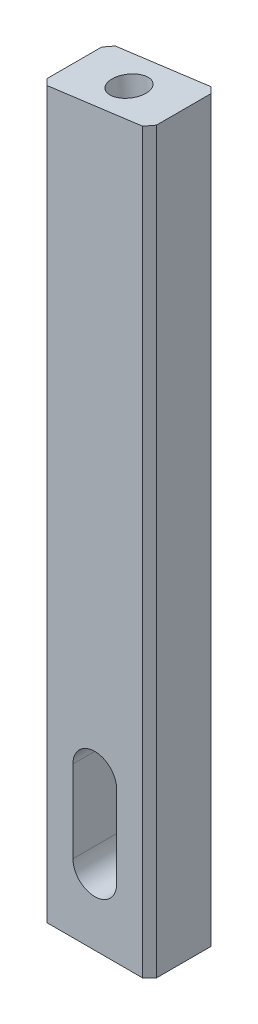
SolidWorks part; units mm, degrees
ref_plane "Front Plane" through (0, 0, 0) normal (0, 0, 1) x (1, 0, 0)
ref_plane "Top Plane" through (0, 0, 0) normal (0, 1, 0) x (1, 0, 0)
ref_plane "Right Plane" through (0, 0, 0) normal (1, 0, 0) x (0, 0, -1)
sketch "Sketch1" plane through (0, 0, 0) normal (0, 0, 1) x (1, 0, 0)
  line L1 (-4, 27) -> (4, 27)
  line L2 (-4, 27) -> (-4, -27)
  line L3 (-4, -27) -> (4, -27)
  line L4 (4, 27) -> (4, -27)
  line L5 (-4, 27) -> (4, -27) construction
  line L6 (-4, -27) -> (4, 27) construction
  point P0 (0, 0)
  dimension "D1" = 8
  dimension "D2" = 54
extrude "Boss-Extrude1" add sketch "Sketch1" along normal mid plane 5
sketch "Sketch2" plane through (0, 0, 2.5) normal (0, 0, 1) x (1, 0, 0)
  line L0 (4, 27) -> (-4, 27) construction
  line L1 (-4, 27) -> (-4, -27) construction
  line L2 (4, 27) -> (-4, 27)
  line L3 (-4, 27) -> (-4, 25.9468)
  line L4 (4, 27) -> (-4, 25.9468)
  dimension "D1" = 7.5
extrude "Cut-Extrude1" cut sketch "Sketch2" against normal through all
hole_wizard "M3 Tapped Hole1" positions "Sketch4" profile "Sketch3" tap size "M3" standard "Gb"
sketch "Sketch4" plane through (-3.4259, 26.0224, 0) normal (-0.1305, 0.9914, 0) x (0.9914, 0.1305, 0)
  line L0 (3.4555, -2.5) -> (3.4555, 2.5) construction
  line L1 (-0.579, -2.5) -> (7.49, -2.5) construction
  line L2 (-0.579, 2.5) -> (7.49, 2.5) construction
  point P0 (3.4555, 0)
sketch "Sketch3" plane through (0, 26.4734, 0) normal (0, 0, 1) x (-0.9914, -0.1305, 0)
  line L0 (0, 0) -> (0, 9.2511)
  line L1 (0, 9.2511) -> (1.25, 8.5)
  line L2 (1.25, 8.5) -> (1.25, 0)
  line L5 (1.25, 0) -> (0, 0)
  line L10 (0, 9.2511) -> (-1.25, 8.5) construction
  line L11 (0, -6.35) -> (0, 107.95) construction
  dimension "螺纹孔钻头直径" = 2.5
  dimension "螺纹孔钻头深度" = 8.5
  dimension "导头角度" = 118
cosmetic thread "Hole Thread1" parameters "D1"=6, "D2"=3
sketch "Sketch5" plane through (0, 0, 2.5) normal (0, 0, 1) x (1, 0, 0)
  line L0 (0, -22) -> (0, -16) construction
  line L1 (-1.6, -22) -> (-1.6, -16)
  line L2 (1.6, -22) -> (1.6, -16)
  line L3 (-4, -27) -> (4, -27) construction
  arc A0 (-1.6, -22) -> (1.6, -22) centre (0, -22) ccw
  arc A1 (1.6, -16) -> (-1.6, -16) centre (0, -16) ccw
  point P3 (0, -19)
  dimension "D1" = 3.2
  dimension "D2" = 6
  dimension "D3" = 8
extrude "Cut-Extrude2" cut sketch "Sketch5" against normal through all
chamfer "Chamfer1" distance 0.5 angle 45 4 edges at (-4, -0.5266, -2.5) (4, 0, -2.5) (4, 0, 2.5) (-4, -0.5266, 2.5)
